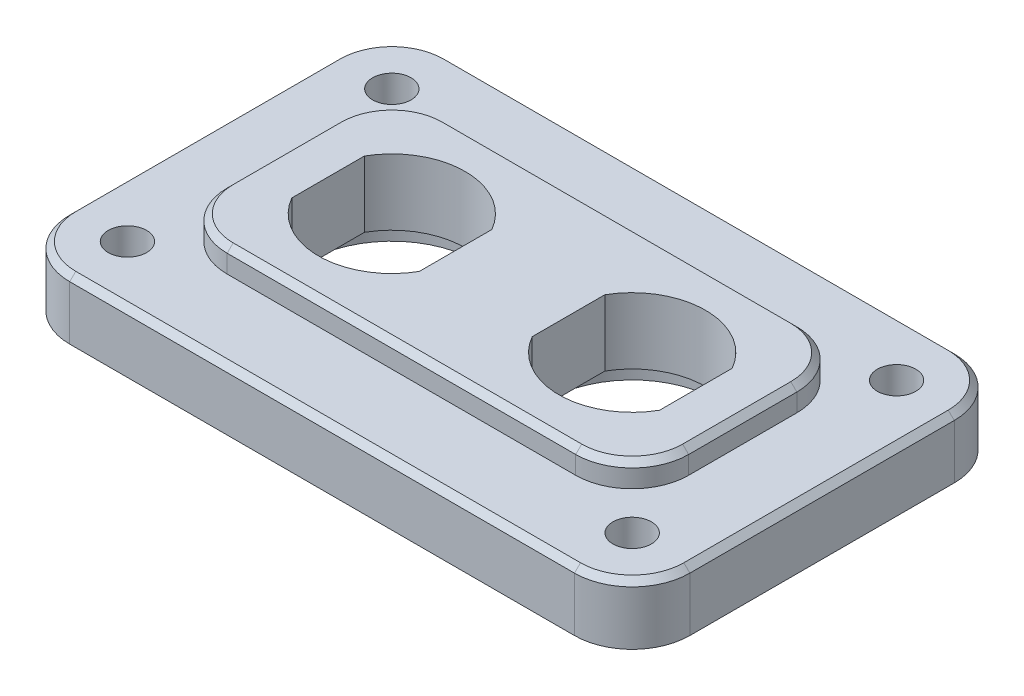
SolidWorks part; units mm, degrees
material "6061-T6 (SS)"
ref_plane "Front" through (0, 0, 0) normal (0, 0, 1) x (1, 0, 0)
ref_plane "Top" through (0, 0, 0) normal (0, 1, 0) x (1, 0, 0)
ref_plane "Right" through (0, 0, 0) normal (1, 0, 0) x (0, 0, -1)
sketch "草图1" plane through (0, 0, 0) normal (1, 0, 0) x (0, 0, -1)
  line L0 (0, 9.6538) -> (0, -9.6538) construction
  line L3 (-15.8, 0) -> (15.8, 0)
  line L4 (15.8, 0) -> (15.8, -5)
  line L5 (15.8, -5) -> (-15.8, -5)
  line L6 (-15.8, 0) -> (-15.8, -5)
  line L9 (16.2924, 0) -> (-16.2924, 0) construction
  dimension "D1" = 5
  dimension "D4" = 31.6
extrude "凸台-拉伸1" add sketch "草图1" along normal mid plane 51.6
sketch "草图2" plane through (0, 0, 0) normal (0, 1, 0) x (1, 0, 0)
  line L0 (-10.7589, 0) -> (10.7589, 0) construction
  line L2 (19.2, 0) -> (-19.2, 0) construction
  line L12 (-19.2, 4.5) -> (-19.2, -4.5)
  line L13 (-14.5, -9.2) -> (14.5, -9.2)
  line L14 (19.2, -4.5) -> (19.2, 4.5)
  line L15 (14.5, 9.2) -> (-14.5, 9.2)
  arc A0 (14.5, 9.2) -> (19.2, 4.5) centre (14.5, 4.5) cw
  arc A1 (19.2, -4.5) -> (14.5, -9.2) centre (14.5, -4.5) cw
  arc A2 (-14.5, -9.2) -> (-19.2, -4.5) centre (-14.5, -4.5) cw
  arc A3 (-14.5, 9.2) -> (-19.2, 4.5) centre (-14.5, 4.5) ccw
  dimension "D2" = 4.7
  dimension "D1" = 18.4
  dimension "D3" = 38.4
extrude "凸台-拉伸2" add sketch "草图2" along normal blind 2
fillet "圆角1" radius 4.8 4 edges at (25.8, -2.5, -15.8) (25.8, -2.5, 15.8) (-25.8, -2.5, -15.8) (-25.8, -2.5, 15.8)
sketch "草图3" plane through (0, -5, 0) normal (0, -1, 0) x (1, 0, 0)
  line L0 (-10, 0) -> (10, 0) construction
  line L1 (-15.3, -3.0199) -> (-15.3, 3.0199)
  line L2 (0, 0) -> (0, 15.2744) construction
  line L3 (15.3, 3.0199) -> (15.3, -3.0199)
  line L4 (-4.7, 3.0199) -> (-4.7, -3.0199)
  line L5 (-10, -6.1) -> (-10, 6.1) construction
  line L6 (4.7, -3.0199) -> (4.7, 3.0199)
  line L7 (10, -6.1) -> (10, 6.1) construction
  line L11 (35.3, 3.0199) -> (35.3, -3.0199) [skipped]
  line L12 (24.7, -3.0199) -> (24.7, 3.0199) [skipped]
  line L13 (30, -6.1) -> (30, 6.1) construction
  circle A1 centre (-10, 0) radius 6.1 construction
  arc A4 (-15.3, -3.0199) -> (-4.7, -3.0199) centre (-10, 0) ccw
  arc A5 (-4.7, 3.0199) -> (-15.3, 3.0199) centre (-10, 0) ccw
  arc A6 (15.3, 3.0199) -> (4.7, 3.0199) centre (10, 0) ccw
  arc A7 (4.7, -3.0199) -> (15.3, -3.0199) centre (10, 0) ccw
  circle A8 centre (10, 0) radius 6.1 construction
  arc A12 (35.3, 3.0199) -> (24.7, 3.0199) centre (30, 0) ccw [skipped]
  arc A13 (24.7, -3.0199) -> (35.3, -3.0199) centre (30, 0) ccw [skipped]
  circle A14 centre (30, 0) radius 6.1 construction
  dimension "D1" = 3
  dimension "D3" = 10.6
  dimension "D5" = 12.2
  dimension "D4" = 10
extrude "切除-拉伸1" cut sketch "草图3" against normal through all
sketch "草图4" plane through (0, -5, 0) normal (0, -1, 0) x (1, 0, 0)
  circle A2 centre (-10, 0) radius 7.1
  circle A3 centre (10, 0) radius 7.1
  arc A6 (15.3, 3.0199) -> (4.7, 3.0199) centre (10, 0) ccw construction
  arc A7 (-4.7, 3.0199) -> (-15.3, 3.0199) centre (-10, 0) ccw construction
  dimension "D1" = 14.2
extrude "切除-拉伸2" cut sketch "草图4" against normal blind 1.5
chamfer "倒角2" distance 0.5 angle 45 16 edges at (24.3941, 0, -14.3941) (24.3941, 0, 14.3941) (0, 0, -15.8) (0, 0, 15.8) (-24.3941, 0, -14.3941) (-24.3941, 0, 14.3941) (17.8234, 2, -7.8234) (0, 2, -9.2) (19.2, 2, 0) (-17.8234, 2, -7.8234) (17.8234, 2, 7.8234) (-19.2, 2, 0) (0, 2, 9.2) (-17.8234, 2, 7.8234) (25.8, 0, 0) (-25.8, 0, 0)
hole_wizard "打孔尺寸(%根据十字)槽半沉头木螺钉的类型1" positions "草图5" profile "草图6" countersink size "M3" standard "GB"
sketch "草图5" plane through (0, -5, 0) normal (0, -1, 0) x (-1, 0, 0)
  line L3 (21, 11) -> (-21, 11) construction
  line L5 (21, -11) -> (-21, -11) construction
  line L6 (21, -11) -> (21, 11) construction
  line L7 (21, 11) -> (-21, -11) construction
  line L8 (-21, -11) -> (-21, 11) construction
  arc A0 (21, -15.8) -> (25.8, -11) centre (21, -11) ccw construction
  arc A1 (25.8, 11) -> (21, 15.8) centre (21, 11) ccw construction
  arc A2 (-25.8, -11) -> (-21, -15.8) centre (-21, -11) ccw construction
  point P0 (21, -11)
  point P16 (-21, -11)
  point P17 (-21, 11)
  point P19 (21, 11)
sketch "草图6" plane through (-21, -5, 11) normal (1, 0, 0) x (0, 0, -1)
  line L0 (0, 0) -> (0, 6.1614)
  line L1 (0, 6.1614) -> (1.6, 5.2)
  line L2 (1.6, 5.2) -> (1.6, 2.1)
  line L3 (1.6, 2.1) -> (3, 0.7)
  line L4 (3, 0.7) -> (3, 0)
  line L6 (3, 0) -> (0, 0)
  line L7 (-1.6, 2.1) -> (-3, 0.7) construction
  line L10 (0, 6.1614) -> (-1.6, 5.2) construction
  line L11 (0, -6.35) -> (0, 107.95) construction
  dimension "孔直径" = 3.2
  dimension "孔深度" = 5.2
  dimension "锥形沉头孔直径" = 6
  dimension "锥形沉头孔角度" = 90
  dimension "导头角度" = 118
  dimension "头间隙" = 0.7
